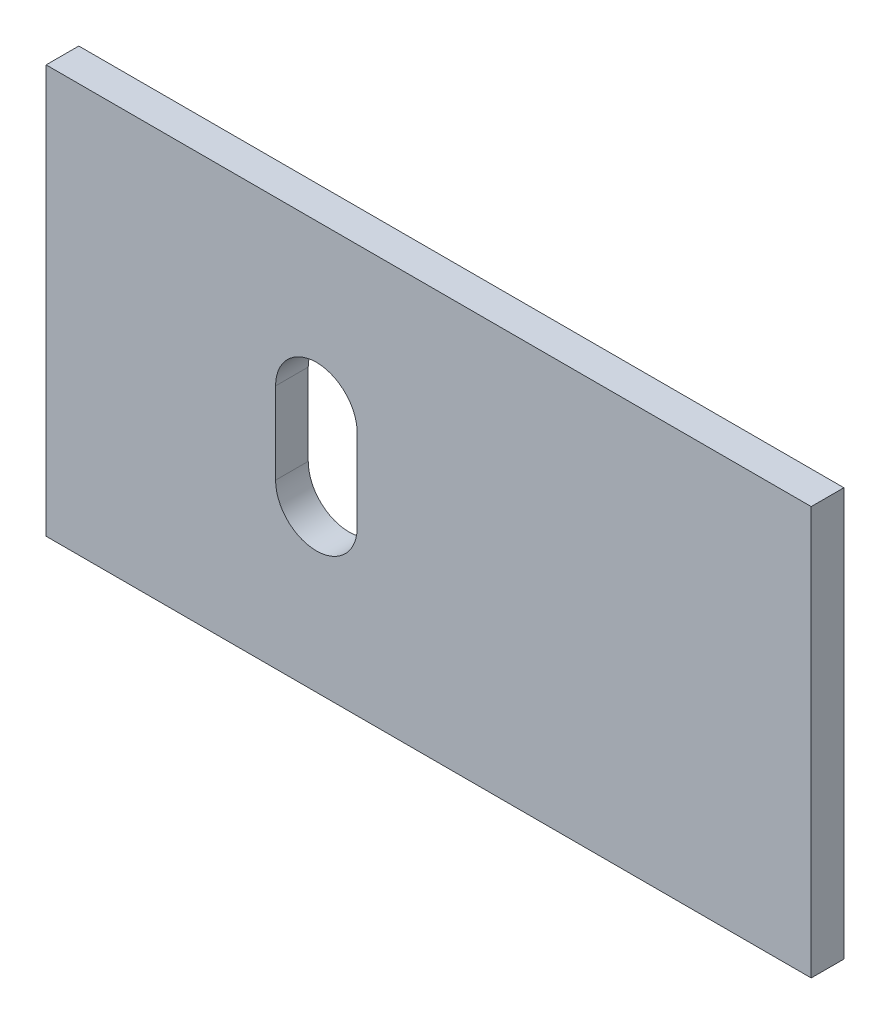
SolidWorks part; units mm, degrees
material "Q235B"
ref_plane "Front Plane" through (0, 0, 0) normal (0, 0, 1) x (1, 0, 0)
ref_plane "Top Plane" through (0, 0, 0) normal (0, 1, 0) x (1, 0, 0)
ref_plane "Right Plane" through (0, 0, 0) normal (1, 0, 0) x (0, 0, -1)
sketch "Sketch1" plane through (0, 0, 0) normal (0, 0, 1) x (1, 0, 0)
  line L0 (9106.7257, 4668.3111) -> (9575.2258, 4668.3111)
  line L1 (9106.7257, 4668.3111) -> (9106.7257, 4418.3111)
  line L2 (9106.7257, 4418.3111) -> (9575.2258, 4418.3111)
  line L3 (9575.2258, 4668.3111) -> (9575.2258, 4418.3111)
  line L4 (9247.2258, 4568.3105) -> (9247.2258, 4518.3113)
  line L5 (9297.2258, 4568.3111) -> (9297.2258, 4518.3111)
  arc A0 (9297.2258, 4568.3111) -> (9247.2258, 4568.3105) centre (9272.2258, 4568.3108) ccw
  arc A1 (9247.2258, 4518.3113) -> (9297.2258, 4518.3111) centre (9272.2258, 4518.3111) ccw
  dimension "D1" = 250
extrude "Boss-Extrude1" add sketch "Sketch1" along normal blind 20
